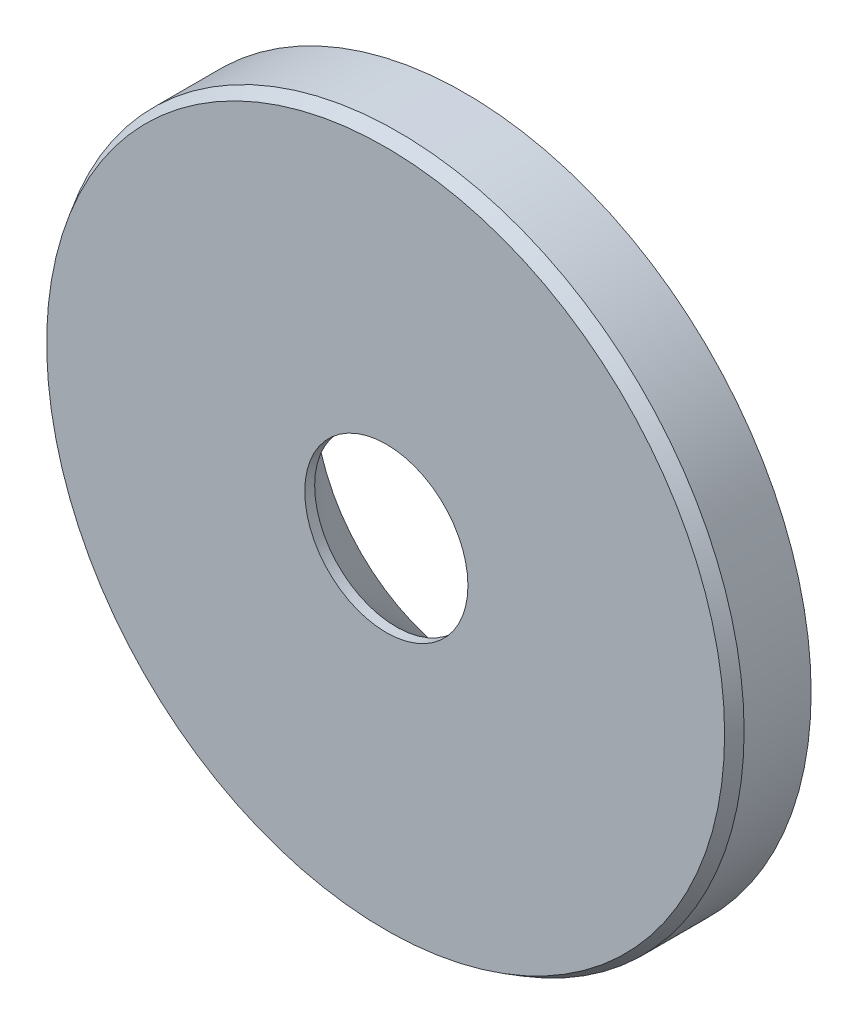
SolidWorks part; units mm, degrees
ref_plane "Front Plane" through (0, 0, 0) normal (0, 0, 1) x (1, 0, 0)
ref_plane "Top Plane" through (0, 0, 0) normal (0, 1, 0) x (1, 0, 0)
ref_plane "Right Plane" through (0, 0, 0) normal (1, 0, 0) x (0, 0, -1)
other "Configuration Table"
sketch "Sketch1" plane through (0, 0, 0) normal (0, 0, 1) x (1, 0, 0)
  circle A0 centre (0, 0) radius 14
  dimension "D1" = 28
extrude "Boss-Extrude1" add sketch "Sketch1" along normal blind 3.5
chamfer "Chamfer1" distance 0.5 angle 30 2 edges at (14, 0, 0) (14, 0, 3.5)
hole_wizard "CSK for M6 Hexagon lobular socket raised CTSK head screws1" positions "3DSketch1" profile "Sketch4" countersink size "M6" standard "GB"
sketch3d "3DSketch1"
  point P0 (0, 0, 0)
  point P3 (0, 0, 0)
  point P5 (0.0285, 0.0173, 0)
sketch "Sketch4" plane through (0.0285, 0.0173, 0) normal (1, 0, 0) x (0, 1, 0)
  line L0 (0, 0) -> (0, 8.4828)
  line L1 (0, 8.4828) -> (3.3, 6.5)
  line L2 (3.3, 6.5) -> (3.3, 3.1)
  line L3 (3.3, 3.1) -> (6.4, 0)
  line L5 (6.4, 0) -> (0, 0)
  line L6 (-3.3, 3.1) -> (-6.4, 0) construction
  line L10 (0, 8.4828) -> (-3.3, 6.5) construction
  line L11 (0, -6.35) -> (0, 107.95) construction
  dimension "孔直径" = 6.6
  dimension "孔深度" = 6.5
  dimension "近端锥形沉头孔直径" = 12.8
  dimension "近端锥形沉头孔角度" = 90
  dimension "导头角度" = 118
